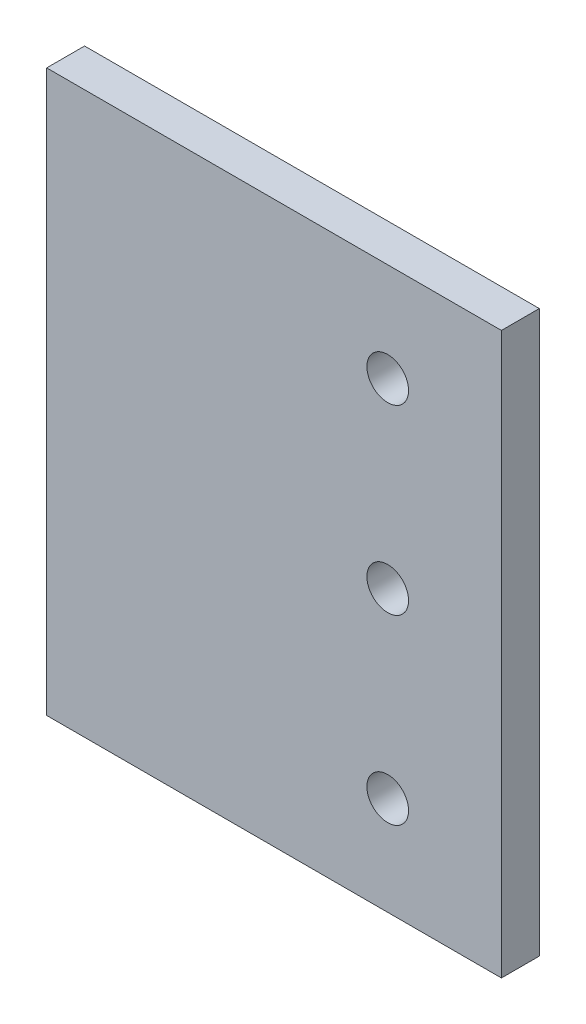
SolidWorks part; units mm, degrees
material "Q235"
ref_plane "Front Plane" through (0, 0, 0) normal (0, 0, 1) x (1, 0, 0)
ref_plane "Top Plane" through (0, 0, 0) normal (0, 1, 0) x (1, 0, 0)
ref_plane "Right Plane" through (0, 0, 0) normal (1, 0, 0) x (0, 0, -1)
sketch "Sketch1" plane through (0, 0, 0) normal (0, 0, 1) x (1, 0, 0)
  line L0 (0, 185) -> (300, 185) construction
  line L1 (0, 0) -> (300, 0)
  line L2 (0, 0) -> (0, 370)
  line L3 (0, 370) -> (300, 370)
  line L4 (300, 0) -> (300, 370)
  line L5 (150, 370) -> (150, 0) construction
  circle A0 centre (225, 305) radius 13.75
  circle A1 centre (225, 185) radius 13.75
  circle A2 centre (225, 65) radius 13.75
  dimension "D3" = 240
  dimension "D4" = 27.5
  dimension "D5" = 75
  dimension "D6" = 120
  dimension "D1" = 300
  dimension "D2" = 370
extrude "Boss-Extrude1" add sketch "Sketch1" along normal blind 25
